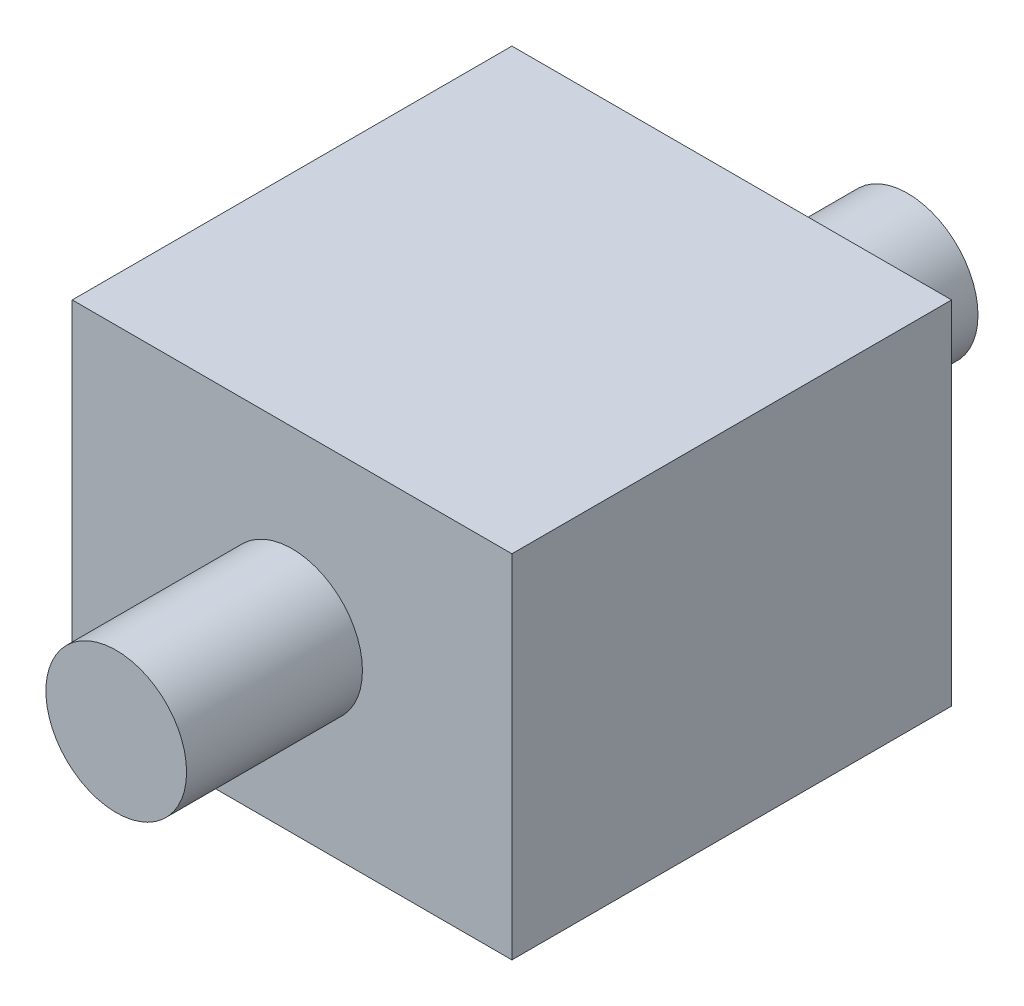
from build123d import *

# Parameters (mm, degrees)
SKETCH1_W           = 25
SKETCH1_H           = 25
BOSS_EXTRUDE1_DEPTH = 20
SKETCH2_R           = 4
BOSS_EXTRUDE2_DEPTH = 10


with BuildPart() as part:
    # Sketch1 → Boss-Extrude1 (new body)
    with BuildSketch(Plane(origin=(0, 0, 0), x_dir=(1, 0, 0), z_dir=(0, 1, 0))):
        Rectangle(SKETCH1_W, SKETCH1_H)
    extrude(amount=BOSS_EXTRUDE1_DEPTH)

    # Sketch2 → Boss-Extrude2 (add)
    with BuildSketch(Plane.XY.offset(12.5)):
        with Locations((0, 10)):
            Circle(SKETCH2_R)
    boss_extrude2 = extrude(amount=BOSS_EXTRUDE2_DEPTH)

    # Mirror1: Boss-Extrude2 across plane
    add(boss_extrude2.mirror(Plane.XY))


solid = part.part
